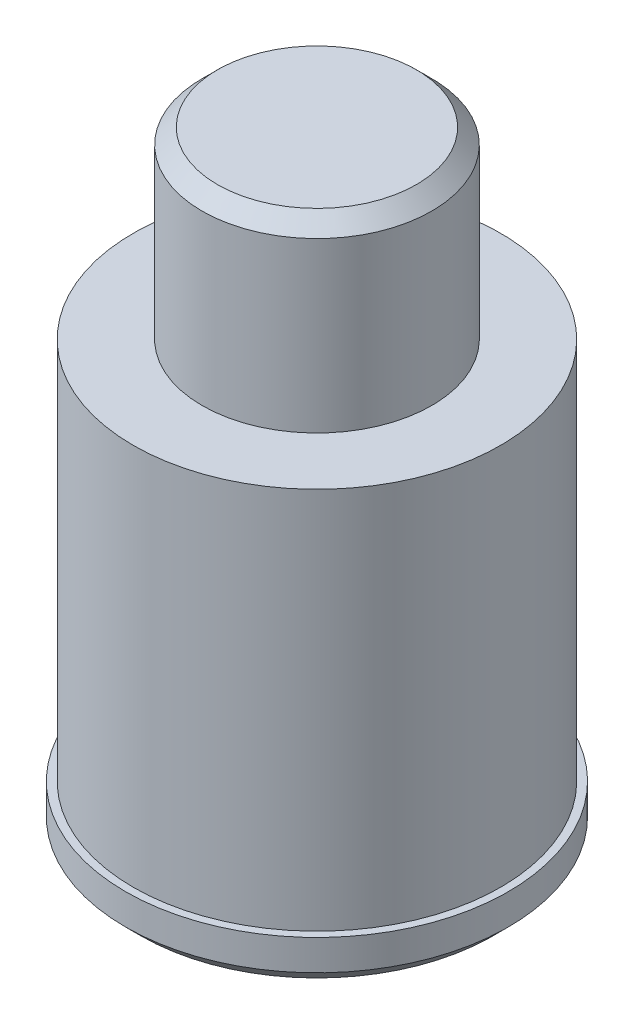
SolidWorks part; units mm, degrees
ref_plane "Front Plane" through (0, 0, 0) normal (0, 0, 1) x (1, 0, 0)
ref_plane "Top Plane" through (0, 0, 0) normal (0, 1, 0) x (1, 0, 0)
ref_plane "Right Plane" through (0, 0, 0) normal (1, 0, 0) x (0, 0, -1)
other "Configuration Table"
sketch "Sketch1" plane through (0, 0, 0) normal (0, 1, 0) x (1, 0, 0)
  circle A0 centre (0, 0) radius 12.5
  dimension "D1" = 25
extrude "Boss-Extrude1" add sketch "Sketch1" along normal blind 3
sketch "Sketch2" plane through (0, 3, 0) normal (0, 1, 0) x (1, 0, 0)
  circle A0 centre (0, 0) radius 12
  dimension "D1" = 24
extrude "Boss-Extrude2" add sketch "Sketch2" along normal blind 25
sketch "Sketch3" plane through (0, 28, 0) normal (0, 1, 0) x (1, 0, 0)
  circle A0 centre (0, 0) radius 7.5
  dimension "D1" = 15
extrude "Boss-Extrude3" add sketch "Sketch3" along normal blind 12
ref_plane "Plane1" through (0, 0, -12) normal (0, 0, -1) x (-1, 0, 0)
sketch "Sketch4" plane through (0, 0, -12) normal (0, 0, -1) x (-1, 0, 0)
  line L0 (0, 23) -> (0, 8) construction
  line L1 (4, 23) -> (4, 8)
  line L2 (-4, 23) -> (-4, 8)
  line L3 (12, 28) -> (-12, 28) construction
  arc A0 (4, 23) -> (-4, 23) centre (0, 23) ccw
  arc A1 (-4, 8) -> (4, 8) centre (0, 8) ccw
  point P3 (0, 15.5)
  dimension "D1" = 8
  dimension "D2" = 15
  dimension "D3" = 5
extrude "Cut-Extrude1" cut sketch "Sketch4" against normal blind 4
chamfer "Chamfer1" distance 1 angle 45 2 edges at (0, 40, 7.5) (0, 0, 12.5)
